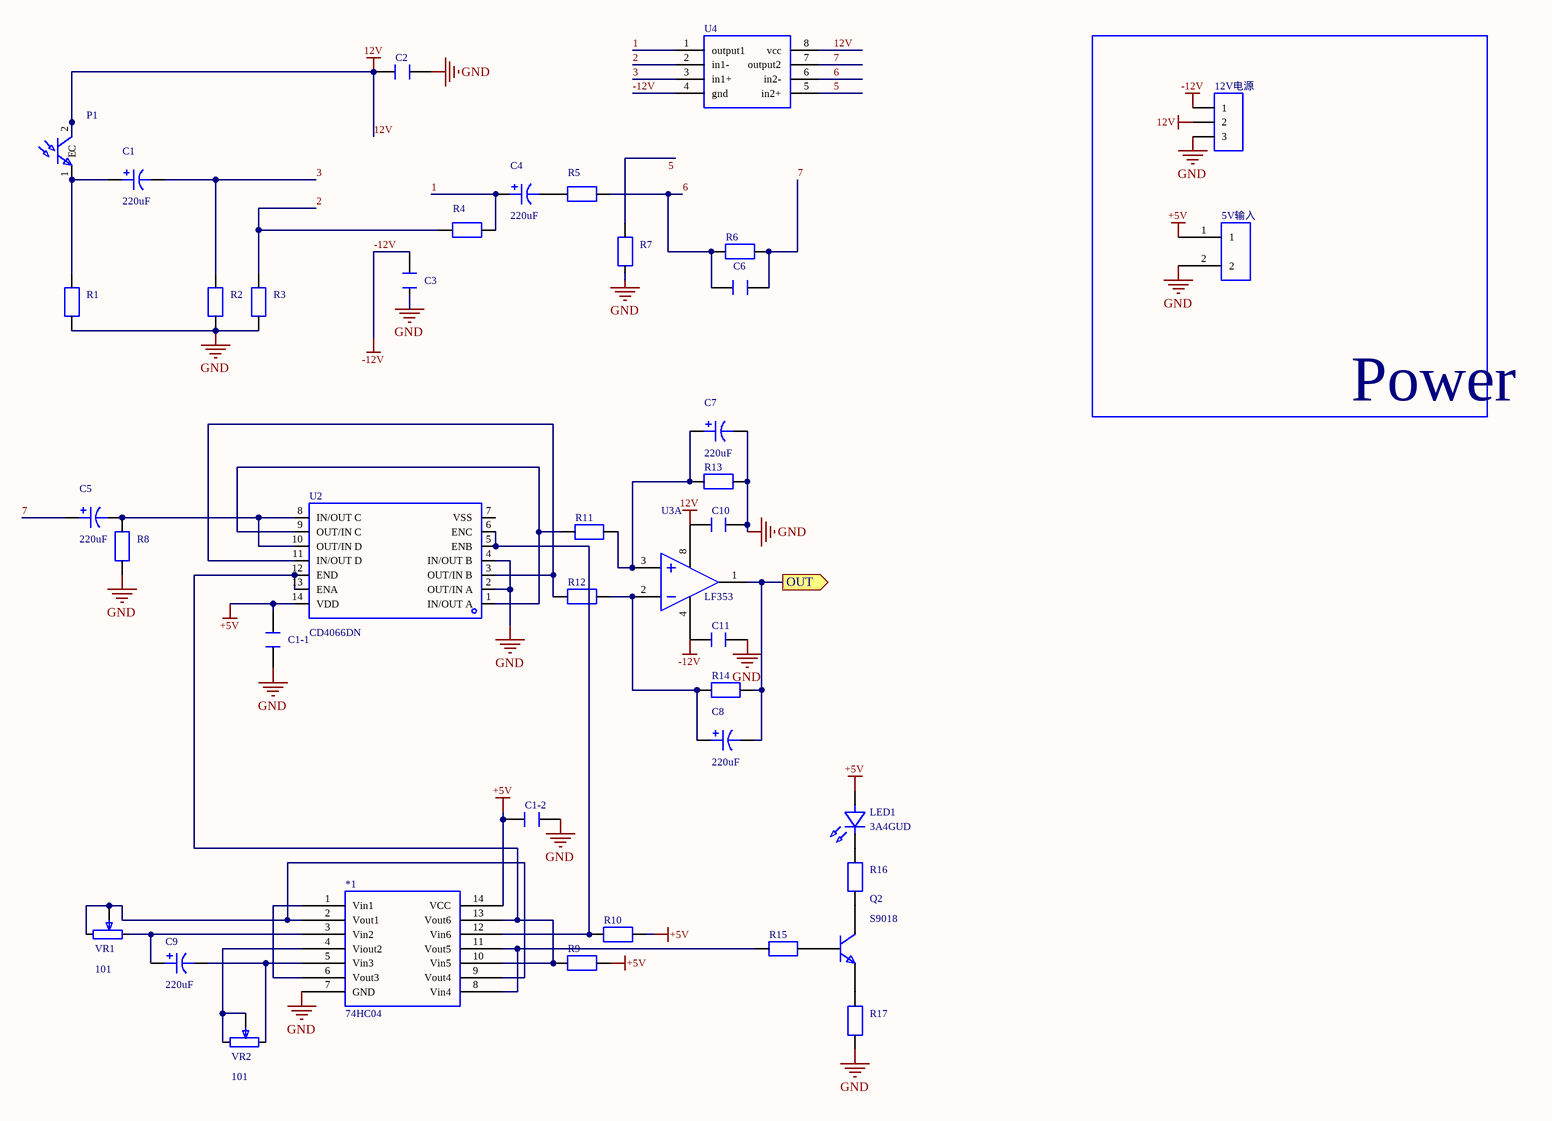
[diagram p0: MISC75397-3.schdoc]
# Altium project MISC75397-2.PrjPcb
1 sheet, 41 parts. Net scope: flat (ports and power ports of the same name join across sheets).
Board file: MISC75397.pcbdoc

## Sheet MISC75397-3.schdoc
size 420 x 297 mm; Version: V1.0; @Project Name: MISC75397; @Page Count: 1; @Update Date: 2026-03-14; @Create Date: 2026-03-14; @Schematic Name: MISC75397; @Page No: 1; @Board Name: MISC75397; @Create Time: 18:26:39; @Update Time: 23:54:28; Size: A4

### Parts
5V输入  5V output  [2INT]  (value not drawn)
12V电源  3PIN  [3PIN]  (value not drawn)
*1  74HC04  [DIP14]
C1  220uF  [CAP-TH_BD6.3-P2.50-D0.5-FD]
C1-1  (no value)  [电容直插]
C1-2  (no value)  [电容直插]
C2  (no value)  [电容直插]
C3  (no value)  [电容直插]
C4  220uF  [CAP-TH_BD6.3-P2.50-D0.5-FD]
C5  220uF  [CAP-TH_BD6.3-P2.50-D0.5-FD]
C6  (no value)  [电容直插]
C7  220uF  [CAP-TH_BD6.3-P2.50-D0.5-FD]
C8  220uF  [CAP-TH_BD6.3-P2.50-D0.5-FD]
C9  220uF  [CAP-TH_BD6.3-P2.50-D0.5-FD]
C10  (no value)  [电容直插]
C11  (no value)  [电容直插]
LED1  3A4GUD  [LED-TH_BD3.5-P2.54-RD-GREEN]
P1  (no value)  [LED_D3.0mm_Horizontal_O1.27mm_Z2.0mm]
Q2  S9018  [TO-92-3_L4.9-W3.7-P1.27-L]
R1  (no value)  [D45-V(直插)]
R2  (no value)  [D45-V(直插)]
R3  (no value)  [D45-V(直插)]
R4  (no value)  [D45-V(直插)]
R5  (no value)  [D45-V(直插)]
R6  (no value)  [D45-V(直插)]
R7  (no value)  [D45-V(直插)]
R8  (no value)  [D45-V(直插)]
R9  (no value)  [D45-V(直插)]
R10  (no value)  [D45-V(直插)]
R11  (no value)  [D45-V(直插)]
R12  (no value)  [D45-V(直插)]
R13  (no value)  [D45-V(直插)]
R14  (no value)  [D45-V(直插)]
R15  (no value)  [D45-V(直插)]
R16  (no value)  [D45-V(直插)]
R17  (no value)  [D45-V(直插)]
U2  CD4066DN  [PDIP-14_L19.3-W6.5-P2.54-LS7.6-BL]
U3  LF353  [DIP-8]  (part A of 2)
U4  (no value)  [DIP-8_L9.9-W6.4-P2.54-LS7.6-BL]
VR1  101  [3296W]
VR2  101  [3296W]

### Blocks framed on the sheet
Power: 5V输入 12V电源

### Ports
OUT (out)

### Nets
12V: 12V电源.2 C2.2 C10.2 P1.2(C) U3.8(V+) U4.8(vcc)
+5V: 5V输入.1 *1.14(VCC) C1-1.2 C1-2.2 LED1.2(A) R9.2 R10.2 U2.14(VDD)
-12V: 12V电源.1 C3.2 C11.2 U3.4(V-) U4.4(gnd)
GND: 5V输入.2 12V电源.3 *1.7(GND) C1-1.1 C1-2.1 C2.1 C3.1 C7.2 C10.1 C11.1 R1.2 R2.2 R3.2 R7.1 R8.2 R13.2 R17.1 U2.2(OUT/IN_A) U2.4(IN/OUT_B)
1: C4.1 R4.1 U4.1(output1)
2: R3.1 R4.2 U4.2(in1-)
3: C1.2 R2.1 U4.3(in1+)
5: R7.2 U4.5(in2+)
6: C6.2 R5.1 R6.1 U4.6(in2-)
7: C5.1 C6.1 R6.2 U4.7(output2)
Net*1_1: *1.1(Vin1) *1.6(Vout3)
Net*1_2: *1.2(Vout1) *1.9(Vout4) VR1.1 VR1.2
Net*1_3: *1.3(Vin2) C9.1 VR1.3
Net*1_4: *1.4(Viout2) VR2.1 VR2.2
Net*1_5: *1.5(Vin3) C9.2 VR2.3
Net*1_8: *1.8(Vin4) *1.11(Vout5) R15.1
Net*1_10: *1.10(Vin5) *1.13(Vout6) R9.1 U2.12(END) U2.13(ENA)
Net*1_12: *1.12(Vin6) R10.1 U2.5(ENB) U2.6(ENC)
NetC1_1: C1.1 P1.1(E) R1.1
NetC4_2: C4.2 R5.2
NetC5_2: C5.2 R8.1 U2.8(IN/OUT_C) U2.10(OUT/IN_D)
NetC7_1: C7.1 R11.2 R13.1 U3.3(IN+)
NetC8_1: C8.1 R12.2 R14.1 U3.2(IN-)
NetC8_2: C8.2 R14.2 U3.1(OUT) ; port OUT
NetLED1_1: LED1.1(C) R16.2
NetQ2_1: Q2.1(E) R17.2
NetQ2_2: Q2.2(B) R15.2
NetQ2_3: Q2.3(C) R16.1
NetR11_1: R11.1 U2.1(IN/OUT_A) U2.9(OUT/IN_C)
NetR12_1: R12.1 U2.3(OUT/IN_B) U2.11(IN/OUT_D)

Not connected (* = marked no-connect by the designer): U2 7(VSS)

### Notes on the sheet
- 2026-03-14
- Schematic
- Board
- Sheet
- P1
- Drawn
- Reviewed
- Project file
- Revision
- Size
- A4
- page 1 Total 1

### Library data of the parts
5V输入 = 2PIN: AddInBom: yes; Device: 2PIN; ConvertToPcb: yes; SymbolName: 2PIN; Origin Footprint 2: 2INT; FootprintName: 2INT
12V电源 = 3PIN: Origin Footprint 2: 1*3PIN; AddInBom: yes; Device: 3PIN; Origin Footprint 3: 3PIN; Origin Footprint 4: 1*3PIN; Origin Footprint 5: 1*3PIN; ConvertToPcb: yes; SymbolName: 1*3PIN; FootprintName: 3PIN
*1 = 74HC04: AddInBom: yes; _: 3; Device: 74HC04; ConvertToPcb: yes; SymbolName: 74HC04; FootprintName: DIP14
C1 C4 C5 C7-C9 = ERG16V220M6X7: Capacitance:220uF;Tolerance:±20%;Rated voltage:16V;Ripple current:300mA@100kHz;Equivalent series resistance(ESR):220mΩ@100kHz;; Manufacturer: JIERR(捷而瑞); AddInBom: yes; ModelId: 983aa343eddc42b59ebb10541a88166e; ModelTransform: 247.99486,248.229,0,90,0,0,0,0,-196.85; Tolerance: ±20%; Voltage Rating: 16V; Pin Spacing: 2.5mm; Lifetime: 2000hrs@105℃; Symbol: ERG16V220M6X7; Device: ERG16V220M6X7; LCSC Part Name: 220uF ±20% 16V; SupplierPart: C47344172; ManufacturerPart: ERG16V220M6X7; Supplier Footprint: 插件,D6.3xL7mm; JLCPCB Part Class: Extended library; Datasheet: https://example.com/datasheet/ERG16V220M6X7/49556613.html; Supplier: LCSC; ConvertToPcb: yes; FootprintName: CAP-TH_BD6.3-P2.50-D0.5-FD; ModelName: CAP-TH_BD6.3-P2.50-D0.5-FD; Value: 220uF; Ripple Current: 300mA@100kHz; Equivalent Series Resistance(ESR): 220mΩ@100kHz; Diameter: 6mm; Height - Seated (Max): 7mm; Operating Temperature: -40℃~+105℃
C1-1 C1-2 C2 C3 C6 C10 C11 = 电容直插: Device: Through-hole capacitor; AddInBom: yes; ModelId: 85437cda0c2b439094ae87a6c0e47ecb; ModelName: Ceramic capacitor; ModelTransform: 222.82,98.42,339.54,0,0,0,0,0,-39.37; ConvertToPcb: yes; SymbolName: Through-hole capacitor; FootprintName: Through-hole capacitor
LED1 = 3A4GUD: Lamp holder type:3mm round lamp holder;Illumination color:Emerald green;Forward voltage(Vf):2.8V~3.2V;Forward current:20mA;Wavelength:520nm~525nm;Lens color:Green lens;Color temperature:-;Luminous intensity:8000mcd~12000mcd;Viewing angle:30°;Operating temperature:-40℃~+85℃;; Manufacturer: Guiguang light(桂光光电); AddInBom: yes; ModelId: 00abdbf2c53742c78999362c055e6c63; ModelTransform: 130.31911,137.754,0,180,0,0,3.15,0,-196.85; Forward Current: 20mA; Peak Wavelength: 525nm; Viewing Angle: 30°; Symbol: 3A4GUD; Device: 3A4GUD; LCSC Part Name: 3mm 绿发翠绿长脚; SupplierPart: C52034646; ManufacturerPart: 3A4GUD; Supplier Footprint: 插件,D=3mm; JLCPCB Part Class: Extended library; Datasheet: https://example.com/datasheet/3A4GUD/54791014.html; Supplier: LCSC; ConvertToPcb: yes; FootprintName: LED-TH_BD3.5-P2.54-RD-GREEN; ModelName: LED-TH_BD3.5-P2.54-RD-GREEN; Lamp Holder Type: 3mm round lamp holder; Illumination Color: Emerald green; Voltage - Forward(Vf): 2.8V~3.2V; Wavelength - Dominant: 520nm~525nm; Lens Color: Green lens; Color Temperature: -; Luminous Intensity: 8000mcd~12000mcd; Operating Temperature: -40℃~+85℃
P1 = LED-3MM-红外接收: Symbol: LED2; Device: LED-3MM-IR receiver; ConvertToPcb: yes; ModelId: 02bfc7c664ed44c69e400cbfd76bc52c; ModelTransform: 135,267.28,229.29,0,0,0,57.5,-122,-100; Value: 红外接收; AddInBom: yes; FootprintName: LED_D3.0mm_Horizontal_O1.27mm_Z2.0mm; ModelName: LED_D3.0mm_Horizontal_O1.27mm_Z2.0mm
Q2 = S9018: Transistor type:NPN;Collector-emitter breakdown voltage(Vceo):18V;Collector current(Ic):50mA;Power(Pd):400mW;Collector cutoff current(Icbo):100nA;Collector-emitter saturation voltage(VCE(sat)@Ic,Ib):500mV@10mA,1mA;DC current gain(hFE@Ic,Vce):97@1mA,5V;Transition frequency(fT):800MHz;Operating temperature:+150℃@(Tj);; Manufacturer: CJ(江苏长电/长晶); AddInBom: yes; ModelId: aafe8e06f2154e7c93506efd0d6632dd; ModelTransform: 180.7872,141.4455,0,0,0,0,0,22.677,-196.85; Transistor Type: NPN; Collector-Emitter Breakdown Voltage (Vceo): 18V; Collector Current (Ic): 50mA; Power Dissipation (Pd): 400mW; Collector Cut-Off Current (Icbo): 100nA; Transition Frequency (fT): 800MHz; Device: S9018; ConvertToPcb: yes; SymbolName: S9018; LCSC Part Name: NPN 18V 50mA H档97-146; SupplierPart: C78893; ManufacturerPart: S9018; Supplier Footprint: TO-92-3; JLCPCB Part Class: Extended Part; Datasheet: https://example.com/upload/public/pdf/source/20160723/1469258983703.pdf; Supplier: LCSC; ModelName: TO-92-3_L4.9-W3.7-P1.27-L; Collector-Emitter Saturation Voltage (VCE(sat)@Ic,Ib): 500mV@10mA,1mA; DC Current Gain (hFE@Ic,Vce): 97@1mA,5V; Operating Temperature: +150℃@(Tj); FootprintName: TO-92-3_L4.9-W3.7-P1.27-L
R1-R17 = 直插电阻: Through-hole resistor; AddInBom: yes; ModelId: 01fe6002a9f04defb2675523a429ba7d; ModelName: Axial_4_0x11_0_Vert; ModelTransform: 992.24408708925,358.65377,210.36173682434887,0,90,90,43.30709,102.3622,299.2126; Device: Through-hole resistor; ConvertToPcb: yes; SymbolName: Through-hole resistor; FootprintName: D45-V (through-hole)
U2 = CD4066DN: Switch circuit:1:1;Channels:4;On-resistance(Ron):125Ω;; Manufacturer: HGSEMI(华冠); AddInBom: yes; ModelId: 7604059b31ae49f98a0332a7cce2343e; ModelTransform: 759.15391,311.417,0,0,0,0,0,0,-129.921; Switch Circuit: 1:1; Number of Channels: 4; Voltage - Supply: 3V~15V; Ron: 125Ω; Propagation Delay (tpd): 15ns; Symbol: CD4066DN; Device: CD4066DN; LCSC Part Name: CD4066DN; SupplierPart: C42406219; ManufacturerPart: CD4066DN; Supplier Footprint: DIP-14; Datasheet: https://example.com/datasheet/CD4066DN/44377199.html; Supplier: LCSC; ConvertToPcb: yes; FootprintName: PDIP-14_L19.3-W6.5-P2.54-LS7.6-BL; ModelName: PDIP-14_L19.3-W6.5-P2.54-LS7.6-BL; Turn-on time: -; Turn-off time: -; Operating Temperature: -20℃~+85℃
U3 = LF353: Relevance: []; AddInBom: yes; ModelId: b25ce56d62334bb48ac4eeaf82c54c81; Device: LF353; LatestRevisionDate: 2023; ConvertToPcb: yes; SymbolName: LF353; FootprintName: DIP-8; ModelName: DIP-8; Publisher: hjh
U4 = lf353: AddInBom: yes; Device: lf353; ConvertToPcb: yes; SymbolName: lf353
VR1 VR2 = 3296: AddInBom: yes; Origin Footprint 2: 103; ModelId: b182808559bb43bda9e7de64b64134cb; Device: 3296; ConvertToPcb: yes; SymbolName: 3296; FootprintName: 3296W; ModelName: 3296W